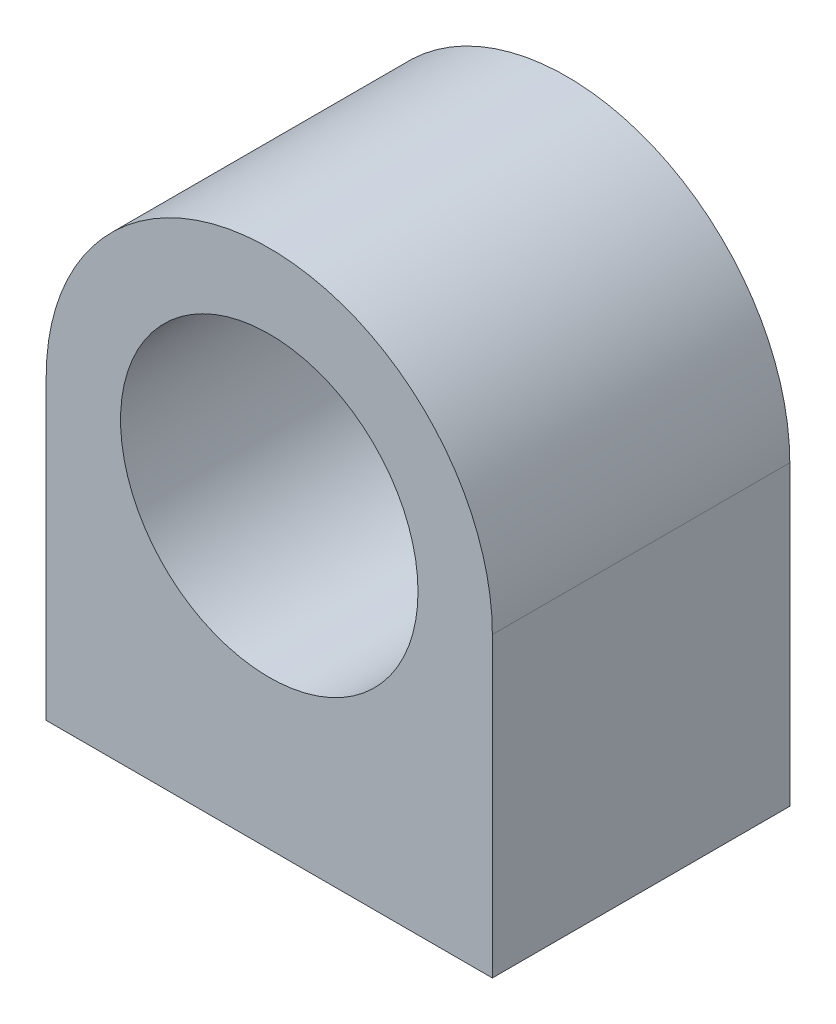
SolidWorks part; units mm, degrees
ref_plane "前视基准面" through (0, 0, 0) normal (0, 0, 1) x (1, 0, 0)
ref_plane "上视基准面" through (0, 0, 0) normal (0, 1, 0) x (1, 0, 0)
ref_plane "右视基准面" through (0, 0, 0) normal (1, 0, 0) x (0, 0, -1)
sketch "草图1" plane through (0, 0, 0) normal (0, 0, 1) x (1, 0, 0)
  line L0 (7.5, 0) -> (7.5, -10)
  line L2 (7.5, -10) -> (-7.5, -10)
  line L3 (-7.5, -10) -> (-7.5, 0)
  circle A0 centre (0, 0) radius 5
  arc A1 (7.5, 0) -> (-7.5, 0) centre (0, 0) ccw
extrude "凸台-拉伸1" add sketch "草图1" along normal blind 10
